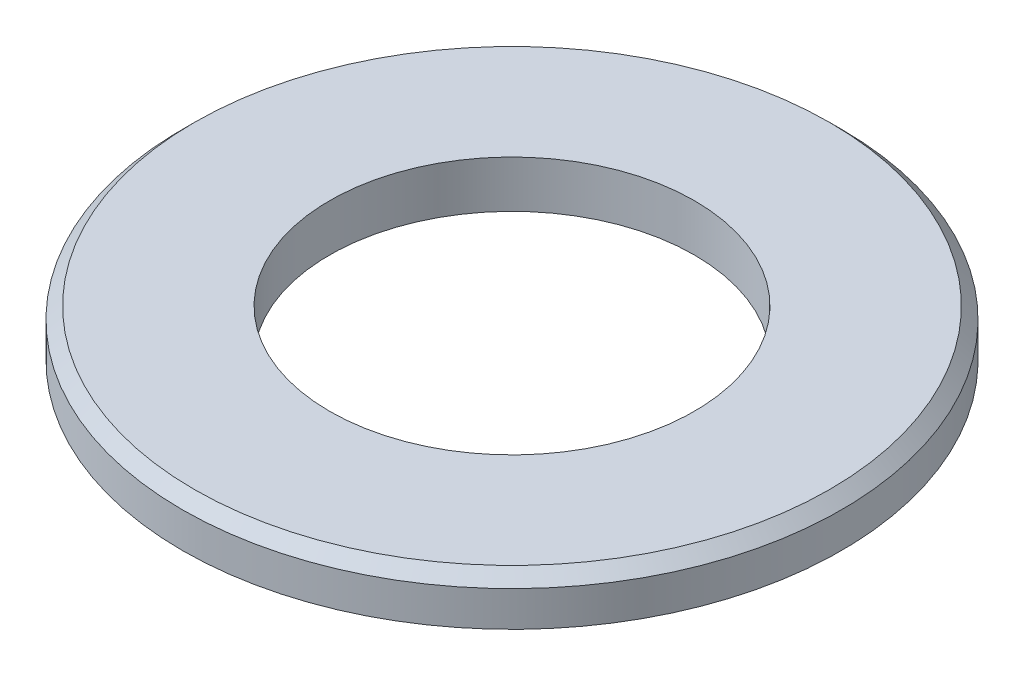
SolidWorks part; units mm, degrees
ref_plane "Plane1" through (0, 0, 0) normal (0, 0, 1) x (1, 0, 0)
ref_plane "Plane2" through (0, 0, 0) normal (0, 1, 0) x (1, 0, 0)
ref_plane "Plane3" through (0, 0, 0) normal (1, 0, 0) x (0, 0, -1)
sketch "dimension sketch" plane through (0, 0, 0) normal (0, 0, 1) x (1, 0, 0)
  line L0 (0, 0) -> (9.1, 0)
  point P3 (4, 0)
  point P4 (56, 0)
  point P5 (31, 0)
sketch "Sketch1" plane through (0, 0, 0) normal (0, 0, 1) x (1, 0, 0)
  line L0 (0, 0) -> (0, 52.7318) construction
  line L1 (-27, 12.6445) -> (-28, 11.6445)
  line L2 (-15.5, 8.6445) -> (-28, 8.6445)
  line L3 (-15.5, 8.6445) -> (-15.5, 12.6445)
  line L4 (-15.5, 12.6445) -> (-27, 12.6445)
  line L5 (-28, 8.6445) -> (-28, 11.6445)
  point P4 (-28, 12.6445)
revolve "Base-Revolve" add sketch "Sketch1" angle 360 about L0
equation "\"h@Sketch1\" = \"h@dimension sketch\""
equation "\"D1@Sketch1\" = \"d1@dimension sketch\" / 2"
equation "\"D2@Sketch1\" = \"d2@dimension sketch\" / 2"
equation "\"D5@Sketch1\" = \"h@Sketch1\" *0.25"
